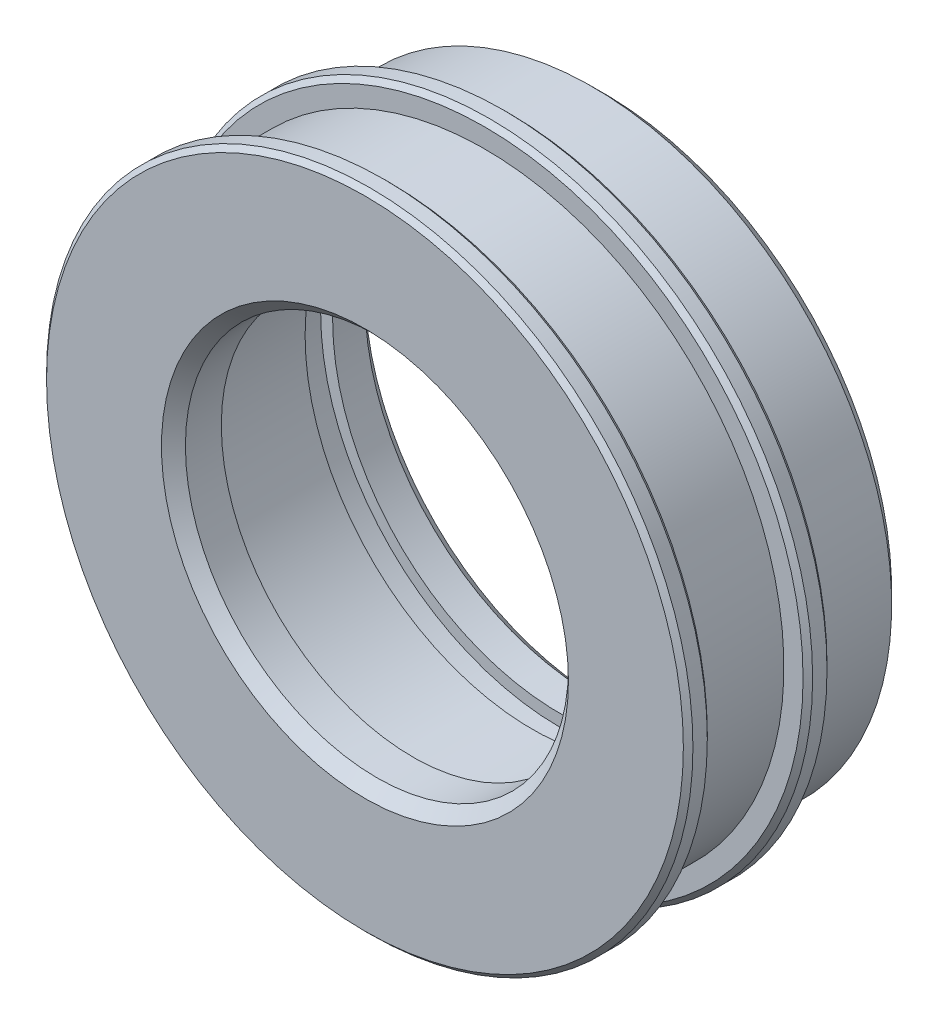
SolidWorks part; units mm, degrees
material "A6061"
ref_plane "Front" through (0, 0, 0) normal (0, 0, 1) x (1, 0, 0)
ref_plane "Top" through (0, 0, 0) normal (0, 1, 0) x (1, 0, 0)
ref_plane "Right" through (0, 0, 0) normal (1, 0, 0) x (0, 0, -1)
sketch "草图1" plane through (0, 0, 0) normal (0, 0, 1) x (1, 0, 0)
  circle A0 centre (0, 0) radius 12.5
  circle A1 centre (0, 0) radius 8
  dimension "D1" = 25
  dimension "D2" = 16
extrude "凸台-拉伸1" add sketch "草图1" along normal blind 4
sketch "草图2" plane through (0, 0, 4) normal (0, 0, 1) x (1, 0, 0)
  circle A0 centre (0, 0) radius 13.5
  circle A1 centre (0, 0) radius 8
  circle A2 centre (0, 0) radius 8 construction
  dimension "D1" = 27
extrude "凸台-拉伸2" add sketch "草图2" along normal blind 1
sketch "草图3" plane through (0, 0, 0) normal (0, 0, -1) x (-1, 0, 0)
  circle A0 centre (0, 0) radius 8
  circle A1 centre (0, 0) radius 13.5
  circle A2 centre (0, 0) radius 13.5 construction
  circle A3 centre (0, 0) radius 8 construction
extrude "凸台-拉伸3" add sketch "草图3" along normal blind 1
sketch "草图4" plane through (0, 0, -1) normal (0, 0, -1) x (-1, 0, 0)
  circle A0 centre (0, 0) radius 9.5
  dimension "D1" = 19
extrude "切除-拉伸1" cut sketch "草图4" against normal blind 4
sketch "草图7" plane through (0, 0, -1) normal (0, 0, -1) x (-1, 0, 0)
  circle A0 centre (0, 0) radius 12.5
  circle A1 centre (0, 0) radius 9.5
  circle A2 centre (0, 0) radius 9.5 construction
  dimension "D1" = 25
extrude "凸台-拉伸4" add sketch "草图7" along normal blind 4
sketch "草图8" plane through (0, 0, -5) normal (0, 0, -1) x (-1, 0, 0)
  circle A0 centre (0, 0) radius 10
  circle A1 centre (0, 0) radius 6
  dimension "D1" = 20
  dimension "D2" = 12
extrude "切除-拉伸2" cut sketch "草图8" along normal blind 1.15 from offset 3 offset against normal yes
chamfer "倒角1" distance 0.5 angle 45 3 edges at (8, 0, 5) (-9.5, 0, -5) (-12.5, 0, -5)
chamfer "倒角2" distance 0.2 angle 45 4 edges at (-13.5, 0, 0) (-13.5, 0, -1) (13.5, 0, 5) (13.5, 0, 4)
